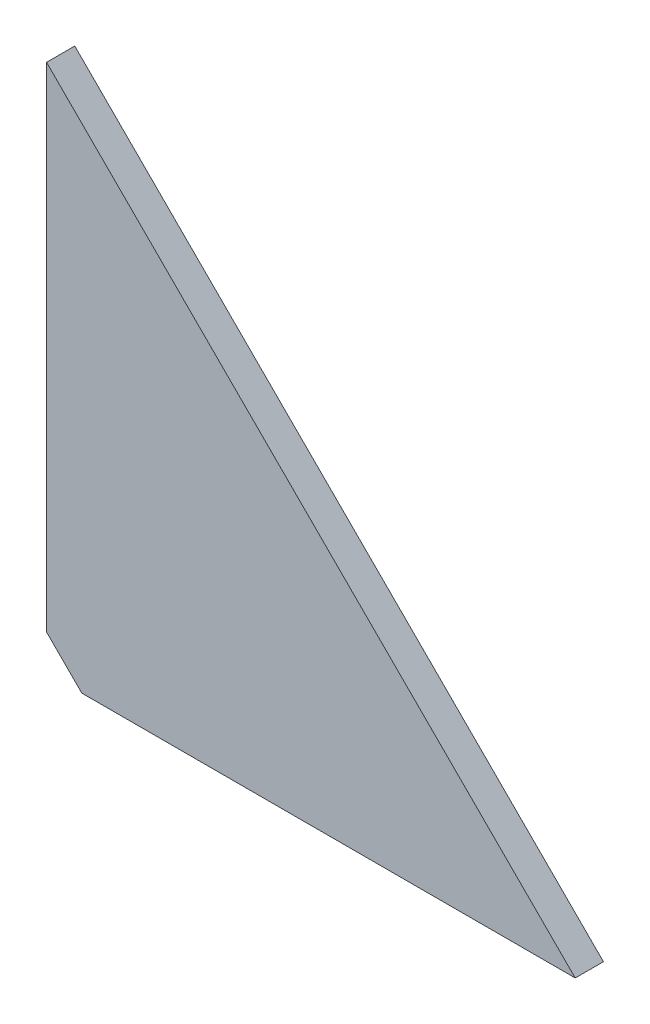
from build123d import *

# Parameters (mm, degrees)
BOSS_EXTRUDE1_DEPTH = 8
CHAMFER1_SIZE       = 20


with BuildPart() as part:
    # Sketch1 → Boss-Extrude1 (new, symmetric)
    with BuildSketch(Plane.XY):
        Polygon((0, 0), (0, 300), (300, 0), align=None)
    extrude(amount=BOSS_EXTRUDE1_DEPTH, both=True)

    # Chamfer1
    chamfer1_edges = [part.edges().sort_by_distance(p)[0] for p in [
        (0, 0, 0),
    ]]
    chamfer(chamfer1_edges, length=CHAMFER1_SIZE)


solid = part.part
